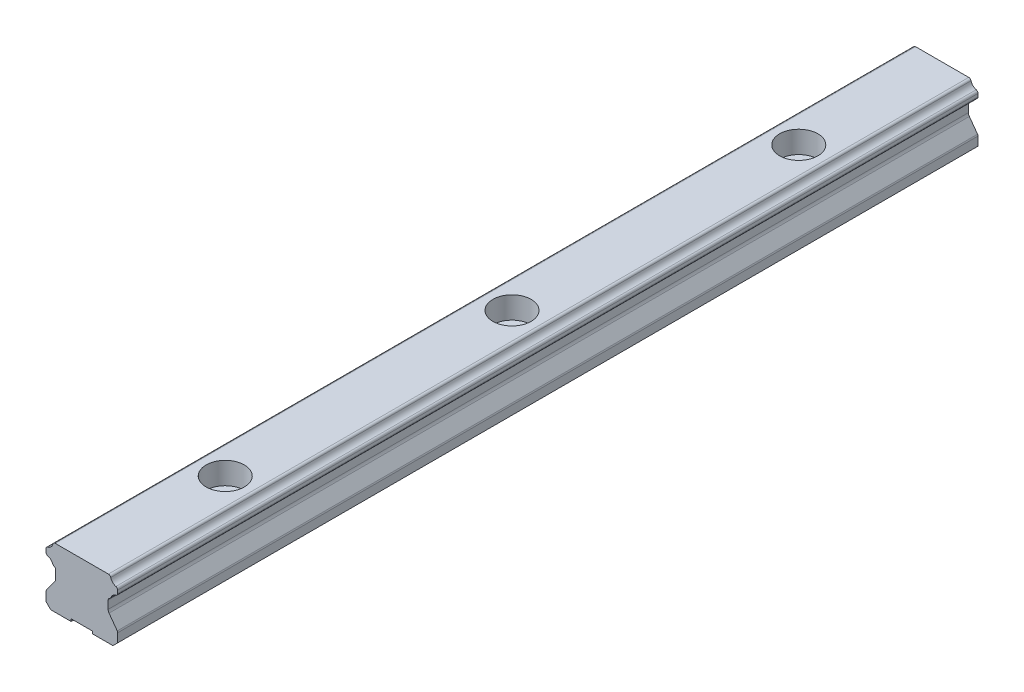
from build123d import *

# Parameters (mm, degrees)
EXTRUDE_1_DEPTH           = 90
HOLE_WIZARD_1_D           = 4.5
HOLE_WIZARD_1_CBORE_D     = 8
HOLE_WIZARD_1_CBORE_DEPTH = 4.6
PATTERN_LINEAR_2_COUNT    = 3
PATTERN_LINEAR_2_PITCH    = 60


with BuildPart() as part:
    # 草图1 → 凸台-拉伸1 (new, symmetric)
    with BuildSketch(Plane.XY):
        with BuildLine():
            Line((-7.5, -9.662591907), (-7.5, -11.5))
            Line((-7.5, -11.5), (-6.5, -12.5))
            Line((-6.5, -12.5), (-2.25, -12.5))
            Line((-2.25, -12.5), (-2.25, -12))
            Line((-2.25, -12), (2.25, -12))
            Line((2.25, -12), (2.25, -12.5))
            Line((2.25, -12.5), (6.5, -12.5))
            Line((6.5, -12.5), (7.5, -11.5))
            Line((7.5, -11.5), (7.5, -9.662591907))
            ThreePointArc((7.5, -9.662591907), (7.475491336, -9.507969821), (7.404368042, -9.368506058))
            Line((7.404368042, -9.368506058), (5.691263916, -7.012987884))
            ThreePointArc((5.691263916, -7.012987884), (5.549017328, -6.734060358), (5.5, -6.424816186))
            Line((5.5, -6.424816186), (5.5, -4.75))
            ThreePointArc((5.5, -4.75), (5.552786405, -4.526393202), (5.7, -4.35))
            Line((5.7, -4.35), (5.9371477, -4.172139225))
            ThreePointArc((5.9371477, -4.172139225), (6.03522297, -4.074688525), (6.102860772, -3.954104425))
            ThreePointArc((6.102860772, -3.954104425), (6.504739846, -3.377744581), (7.12499999, -3.047631248))
            ThreePointArc((7.12499999, -3.047631248), (7.395284704, -2.869694549), (7.5, -2.563508327))
            Line((7.5, -2.563508327), (7.5, -1.936491673))
            ThreePointArc((7.5, -1.936491673), (7.395284705, -1.630305452), (7.124999991, -1.452368753))
            ThreePointArc((7.124999991, -1.452368753), (6.439339825, -1.060660169), (6.047631245, -0.375))
            ThreePointArc((6.047631245, -0.375), (5.869694545, -0.104715292), (5.563508327, 0))
            Line((5.563508327, 0), (-5.563508327, 0))
            ThreePointArc((-5.563508327, 0), (-5.869694545, -0.104715292), (-6.047631245, -0.375))
            ThreePointArc((-6.047631245, -0.375), (-6.439339824, -1.060660168), (-7.12499999, -1.452368752))
            ThreePointArc((-7.12499999, -1.452368752), (-7.395284704, -1.630305451), (-7.5, -1.936491673))
            Line((-7.5, -1.936491673), (-7.5, -2.563508327))
            ThreePointArc((-7.5, -2.563508327), (-7.395284705, -2.869694548), (-7.124999991, -3.047631247))
            ThreePointArc((-7.124999991, -3.047631247), (-6.504739849, -3.377744578), (-6.102860775, -3.954104419))
            ThreePointArc((-6.102860775, -3.954104419), (-6.035222972, -4.074688523), (-5.9371477, -4.172139225))
            Line((-5.9371477, -4.172139225), (-5.7, -4.35))
            ThreePointArc((-5.7, -4.35), (-5.552786405, -4.526393202), (-5.5, -4.75))
            Line((-5.5, -4.75), (-5.5, -6.424816186))
            ThreePointArc((-5.5, -6.424816186), (-5.549017328, -6.734060358), (-5.691263916, -7.012987884))
            Line((-5.691263916, -7.012987884), (-7.404368042, -9.368506058))
            ThreePointArc((-7.404368042, -9.368506058), (-7.475491336, -9.507969821), (-7.5, -9.662591907))
        make_face()
    extrude(amount=EXTRUDE_1_DEPTH, both=True)

    # 打孔尺寸(%根据)内六角圆柱头螺钉的类型1 (through all)
    with Locations(Plane(origin=(0, 0, -60), x_dir=(0, 0, 1), z_dir=(0, 1, 0))):
        with Locations((0, 0)):
            hole_wizard_1 = CounterBoreHole(HOLE_WIZARD_1_D / 2, HOLE_WIZARD_1_CBORE_D / 2, HOLE_WIZARD_1_CBORE_DEPTH)

    # 阵列(线性)2: 打孔尺寸(%根据)内六角圆柱头螺钉的类型1 ×3
    with Locations(*[(0, 0, i * PATTERN_LINEAR_2_PITCH) for i in range(1, PATTERN_LINEAR_2_COUNT)]):
        add(hole_wizard_1, mode=Mode.SUBTRACT)


solid = part.part
